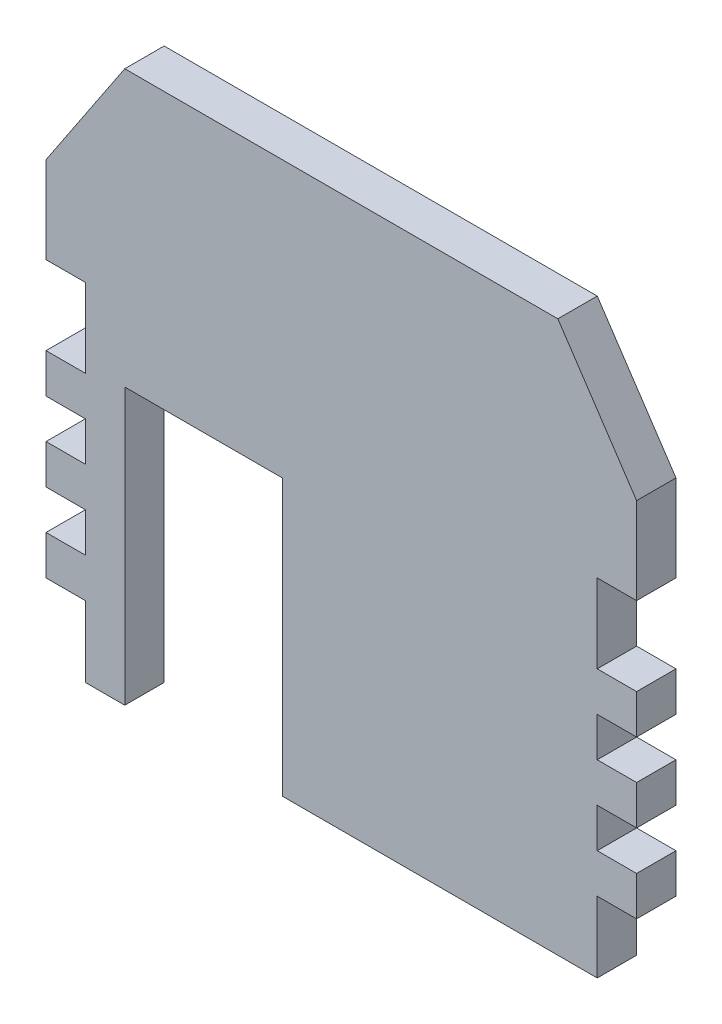
from build123d import *

# Parameters (mm, degrees)
SKETCH1_W           = 75
SKETCH1_H           = 75
BOSS_EXTRUDE1_DEPTH = 5
CUT_EXTRUDE1_DEPTH  = 5
SKETCH3_W           = 20
SKETCH3_H           = 40
CUT_EXTRUDE2_DEPTH  = 5
CUT_EXTRUDE3_REACH  = 55.268
SKETCH4_W           = 5
SKETCH4_H           = 14
SKETCH4_H_2         = 5
SKETCH4_H_3         = 10
CUT_EXTRUDE4_REACH  = 55.268
SKETCH5_W           = 5
SKETCH5_H           = 5
SKETCH5_H_2         = 14
SKETCH5_H_3         = 10
SKETCH7_W           = 65
SKETCH7_H           = 5
CUT_EXTRUDE5_DEPTH  = 10


with BuildPart() as part:
    # Sketch1 → Boss-Extrude1 (new body)
    with BuildSketch(Plane.XY):
        Rectangle(SKETCH1_W, SKETCH1_H)
    extrude(amount=BOSS_EXTRUDE1_DEPTH)

    # Sketch2 → Cut-Extrude1 (cut)
    with BuildSketch(Plane.XY.offset(5)):
        Polygon((-27.5, 37.5), (-37.5, 22.5), (-37.5, 37.5), align=None)
        Polygon((37.5, 37.5), (27.5, 37.5), (37.5, 22.5), align=None)
    extrude(amount=-CUT_EXTRUDE1_DEPTH, mode=Mode.SUBTRACT)

    # Sketch3 → Cut-Extrude2 (cut)
    with BuildSketch(Plane.XY.offset(5)):
        with Locations((-17.5, -17.5)):
            Rectangle(SKETCH3_W, SKETCH3_H)
    extrude(amount=-CUT_EXTRUDE2_DEPTH, mode=Mode.SUBTRACT)

    # Sketch4 → Cut-Extrude3 (cut, up to next)
    with BuildSketch(Plane.XY.offset(5), mode=Mode.PRIVATE) as cut_extrude3_sk1:
        with Locations((-35, -30.5)):
            Rectangle(SKETCH4_W, SKETCH4_H)
    cut_extrude3_tool1 = extrude(cut_extrude3_sk1.sketch, amount=-CUT_EXTRUDE3_REACH, mode=Mode.PRIVATE) & part.part
    # Sketch4 → Cut-Extrude3 (cut, up to next)
    with BuildSketch(Plane.XY.offset(5), mode=Mode.PRIVATE) as cut_extrude3_sk2:
        with Locations((-35, -16)):
            Rectangle(SKETCH4_W, SKETCH4_H_2)
    cut_extrude3_tool2 = extrude(cut_extrude3_sk2.sketch, amount=-CUT_EXTRUDE3_REACH, mode=Mode.PRIVATE) & part.part
    # Sketch4 → Cut-Extrude3 (cut, up to next)
    with BuildSketch(Plane.XY.offset(5), mode=Mode.PRIVATE) as cut_extrude3_sk3:
        with Locations((-35, -6)):
            Rectangle(SKETCH4_W, SKETCH4_H_2)
    cut_extrude3_tool3 = extrude(cut_extrude3_sk3.sketch, amount=-CUT_EXTRUDE3_REACH, mode=Mode.PRIVATE) & part.part
    # Sketch4 → Cut-Extrude3 (cut, up to next)
    with BuildSketch(Plane.XY.offset(5), mode=Mode.PRIVATE) as cut_extrude3_sk4:
        with Locations((-35, 6.5)):
            Rectangle(SKETCH4_W, SKETCH4_H_3)
    cut_extrude3_tool4 = extrude(cut_extrude3_sk4.sketch, amount=-CUT_EXTRUDE3_REACH, mode=Mode.PRIVATE) & part.part
    add(cut_extrude3_tool1.solids().sort_by_distance((-35, -30.5, 5))[0], mode=Mode.SUBTRACT)
    add(cut_extrude3_tool2.solids().sort_by_distance((-35, -16, 5))[0], mode=Mode.SUBTRACT)
    add(cut_extrude3_tool3.solids().sort_by_distance((-35, -6, 5))[0], mode=Mode.SUBTRACT)
    add(cut_extrude3_tool4.solids().sort_by_distance((-35, 6.5, 5))[0], mode=Mode.SUBTRACT)

    # Sketch5 → Cut-Extrude4 (cut, up to next)
    with BuildSketch(Plane.XY.offset(5), mode=Mode.PRIVATE) as cut_extrude4_sk1:
        with Locations((35, -16)):
            Rectangle(SKETCH5_W, SKETCH5_H)
    cut_extrude4_tool1 = extrude(cut_extrude4_sk1.sketch, amount=-CUT_EXTRUDE4_REACH, mode=Mode.PRIVATE) & part.part
    # Sketch5 → Cut-Extrude4 (cut, up to next)
    with BuildSketch(Plane.XY.offset(5), mode=Mode.PRIVATE) as cut_extrude4_sk2:
        with Locations((35, -6)):
            Rectangle(SKETCH5_W, SKETCH5_H)
    cut_extrude4_tool2 = extrude(cut_extrude4_sk2.sketch, amount=-CUT_EXTRUDE4_REACH, mode=Mode.PRIVATE) & part.part
    # Sketch5 → Cut-Extrude4 (cut, up to next)
    with BuildSketch(Plane.XY.offset(5), mode=Mode.PRIVATE) as cut_extrude4_sk3:
        with Locations((35, -30.5)):
            Rectangle(SKETCH5_W, SKETCH5_H_2)
    cut_extrude4_tool3 = extrude(cut_extrude4_sk3.sketch, amount=-CUT_EXTRUDE4_REACH, mode=Mode.PRIVATE) & part.part
    # Sketch5 → Cut-Extrude4 (cut, up to next)
    with BuildSketch(Plane.XY.offset(5), mode=Mode.PRIVATE) as cut_extrude4_sk4:
        with Locations((35, 6.5)):
            Rectangle(SKETCH5_W, SKETCH5_H_3)
    cut_extrude4_tool4 = extrude(cut_extrude4_sk4.sketch, amount=-CUT_EXTRUDE4_REACH, mode=Mode.PRIVATE) & part.part
    add(cut_extrude4_tool1.solids().sort_by_distance((35, -16, 5))[0], mode=Mode.SUBTRACT)
    add(cut_extrude4_tool2.solids().sort_by_distance((35, -6, 5))[0], mode=Mode.SUBTRACT)
    add(cut_extrude4_tool3.solids().sort_by_distance((35, -30.5, 5))[0], mode=Mode.SUBTRACT)
    add(cut_extrude4_tool4.solids().sort_by_distance((35, 6.5, 5))[0], mode=Mode.SUBTRACT)

    # Sketch7 → Cut-Extrude5 (cut)
    with BuildSketch(Plane.XY.offset(5)):
        with Locations((0, -35)):
            Rectangle(SKETCH7_W, SKETCH7_H)
    extrude(amount=-CUT_EXTRUDE5_DEPTH, mode=Mode.SUBTRACT)


solid = part.part
